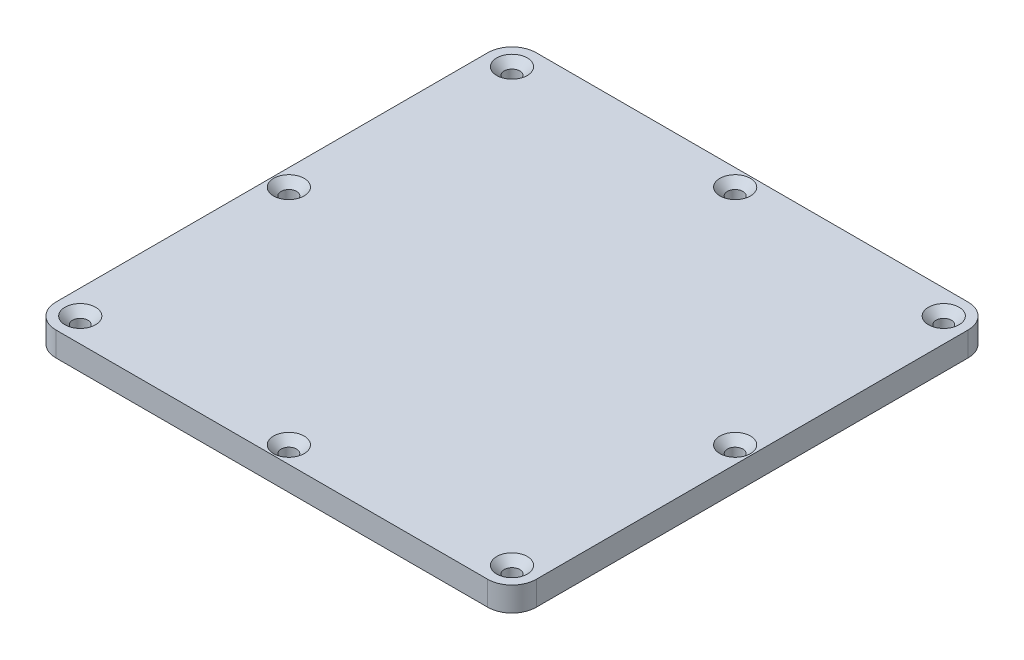
from build123d import *

# Parameters (mm, degrees)
SKETCH1_W                                       = 99
SKETCH1_H                                       = 99
BOSS_EXTRUDE1_DEPTH                             = 5
FILLET1_R                                       = 5
CSK_FOR_M3_FLAT_HEAD_MACHINE_SCREW1_D           = 3.2
CSK_FOR_M3_FLAT_HEAD_MACHINE_SCREW1_DEPTH       = 8.5
CSK_FOR_M3_FLAT_HEAD_MACHINE_SCREW1_CSINK_D     = 6.3
CSK_FOR_M3_FLAT_HEAD_MACHINE_SCREW1_CSINK_ANGLE = 90
CSK_FOR_M3_FLAT_HEAD_MACHINE_SCREW1_TIP         = 0.96137699


with BuildPart() as part:
    # Sketch1 → Boss-Extrude1 (new body)
    with BuildSketch(Plane(origin=(0, 0, 0), x_dir=(1, 0, 0), z_dir=(0, 1, 0))):
        Rectangle(SKETCH1_W, SKETCH1_H)
    extrude(amount=BOSS_EXTRUDE1_DEPTH)

    # Fillet1
    fillet1_edges = [part.edges().sort_by_distance(p)[0] for p in [
        (49.5, 2.5, 49.5),
        (-49.5, 2.5, 49.5),
        (-49.5, 2.5, -49.5),
        (49.5, 2.5, -49.5),
    ]]
    fillet(fillet1_edges, radius=FILLET1_R)

    # CSK for M3 Flat Head Machine Screw1
    with Locations(Plane(origin=(0, 5, 0), x_dir=(1, 0, 0), z_dir=(0, 1, 0))):
        with Locations((-44.5, 44.5), (44.5, 44.5), (0, 46), (-46, 0), (-44.5, -44.5), (0, -46), (44.5, -44.5), (46, 0)):
            CounterSinkHole(CSK_FOR_M3_FLAT_HEAD_MACHINE_SCREW1_D / 2, CSK_FOR_M3_FLAT_HEAD_MACHINE_SCREW1_CSINK_D / 2, depth=CSK_FOR_M3_FLAT_HEAD_MACHINE_SCREW1_DEPTH, counter_sink_angle=CSK_FOR_M3_FLAT_HEAD_MACHINE_SCREW1_CSINK_ANGLE)
            with Locations((0, 0, -(CSK_FOR_M3_FLAT_HEAD_MACHINE_SCREW1_DEPTH + CSK_FOR_M3_FLAT_HEAD_MACHINE_SCREW1_TIP / 2))):  # 118° drill point
                Cone(0, CSK_FOR_M3_FLAT_HEAD_MACHINE_SCREW1_D / 2, CSK_FOR_M3_FLAT_HEAD_MACHINE_SCREW1_TIP, mode=Mode.SUBTRACT)


solid = part.part
